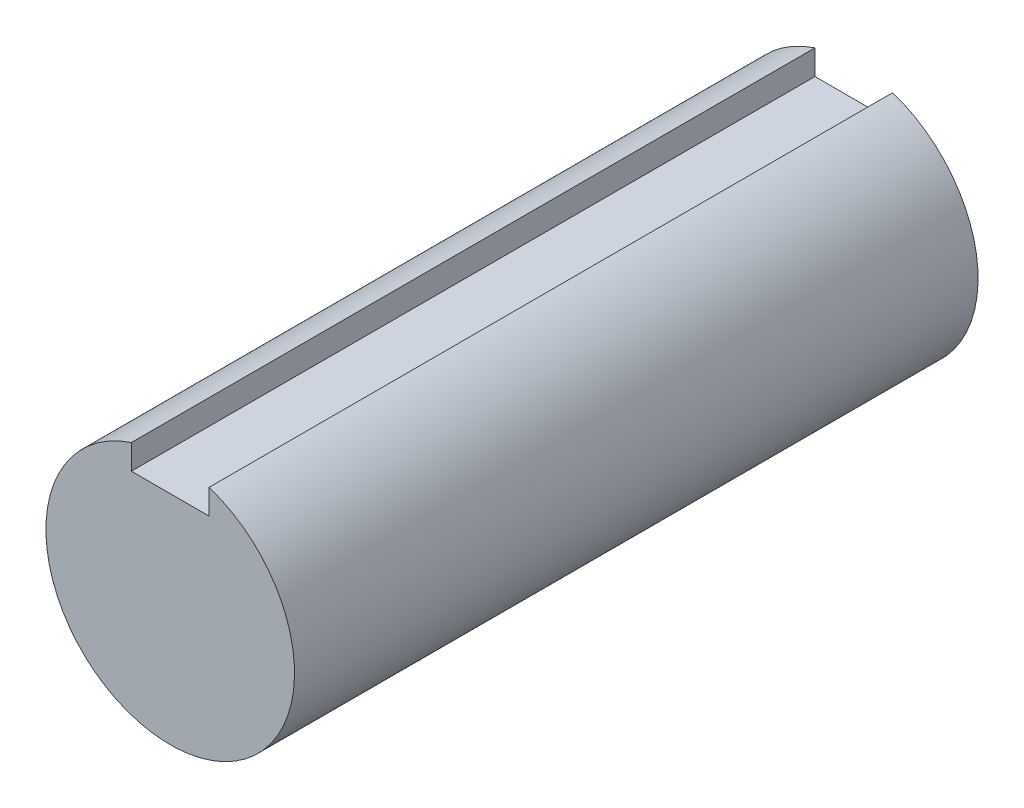
from build123d import *

# Parameters (mm, degrees)
BOSS_EXTRUDE1_DEPTH = 44


with BuildPart() as part:
    # Sketch1 → Boss-Extrude1 (new body)
    with BuildSketch(Plane.XY):
        with BuildLine():
            Line((-271.5, 6), (-271.5, 7.599342077))
            ThreePointArc((-271.5, 7.599342077), (-274, -8), (-276.5, 7.599342077))
            Line((-276.5, 7.599342077), (-276.5, 6))
            Line((-276.5, 6), (-271.5, 6))
        make_face()
    extrude(amount=-BOSS_EXTRUDE1_DEPTH)


solid = part.part
